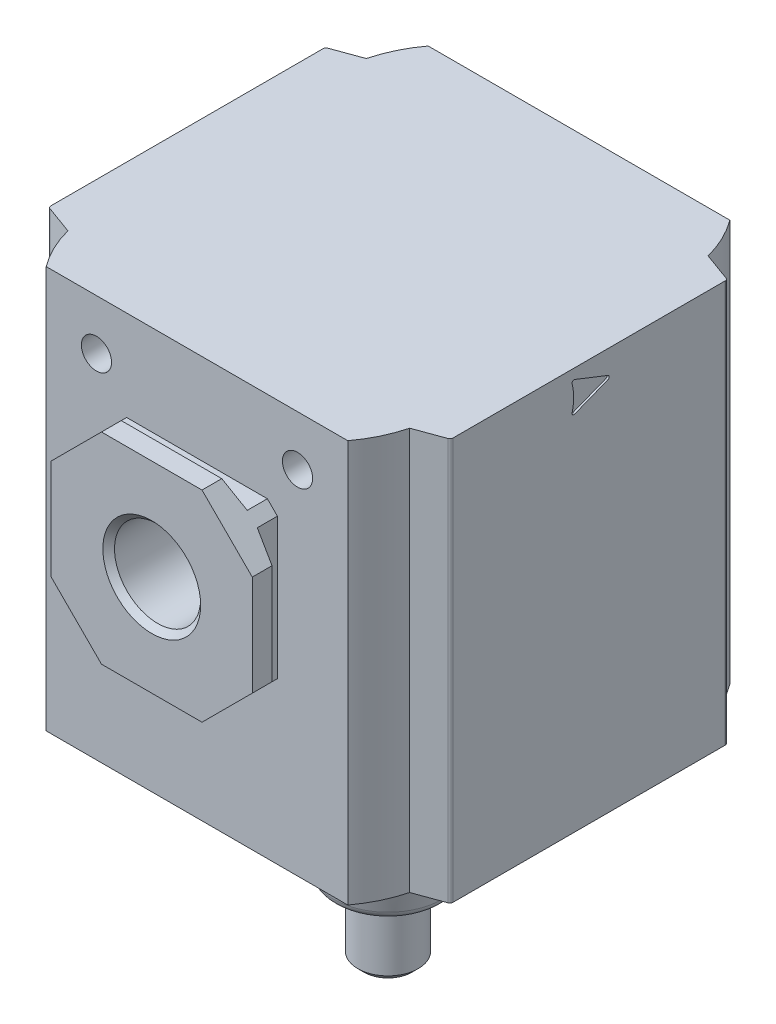
from build123d import *

# Parameters (mm, degrees)
EXTRUDE_1_DEPTH          = 40
EXTRUDE_2_DEPTH          = 40
EXTRUDE_3_DEPTH          = 40
EXTRUDE_4_DEPTH          = 2
EXTRUDE_5_DEPTH          = 2.5
CUT_EXTRUDE_1_DEPTH      = 10
CUT_EXTRUDE_1_DEPTH_BACK = 10
CUT_EXTRUDE_2_DEPTH      = 10
CUT_EXTRUDE_2_DEPTH_BACK = 10
CUT_EXTRUDE_3_DEPTH      = 10
CUT_EXTRUDE_3_DEPTH_BACK = 10
CUT_EXTRUDE_4_DEPTH      = 10
CUT_EXTRUDE_4_DEPTH_BACK = 10
EXTRUDE_6_DEPTH          = 2
EXTRUDE_7_DEPTH          = 2.5
CUT_EXTRUDE_5_DEPTH      = 10
CUT_EXTRUDE_5_DEPTH_BACK = 10
CUT_EXTRUDE_6_DEPTH      = 10
CUT_EXTRUDE_6_DEPTH_BACK = 10
CUT_EXTRUDE_7_DEPTH      = 10
CUT_EXTRUDE_7_DEPTH_BACK = 10
CUT_EXTRUDE_8_DEPTH      = 10
CUT_EXTRUDE_8_DEPTH_BACK = 10
SKETCH_18_R              = 1.5
CUT_EXTRUDE_9_DEPTH      = 4
SKETCH_19_R              = 1.5
CUT_EXTRUDE_10_DEPTH     = 4
CUT_EXTRUDE_START        = -4
SKETCH_20_R              = 1.5
CUT_EXTRUDE_11_DEPTH     = 4
SKETCH_21_R              = 1.5
CUT_EXTRUDE_12_DEPTH     = 4
SKETCH_22_W              = 16.9585
SKETCH_22_H              = 11
CUT_EXTRUDE_13_DEPTH     = 0.2
CUT_EXTRUDE_START_2      = 0.2
CUT_EXTRUDE_14_DEPTH     = 0.2


with BuildPart() as part:
    # 草图1 → 凸台-拉伸1 (new body)
    with BuildSketch(Plane(origin=(0, 0, 0), x_dir=(1, 0, 0), z_dir=(0, 1, 0))):
        with BuildLine():
            Line((-17, 14.841910703), (-17, -14.841910703))
            ThreePointArc((-17, -14.841910703), (-16.201733132, -17.017987001), (-15, -19))
            Line((-15, -19), (15, -19))
            ThreePointArc((15, -19), (16.201733132, -17.017987001), (17, -14.841910703))
            Line((17, -14.841910703), (17, 14.841910703))
            ThreePointArc((17, 14.841910703), (16.201733132, 17.017987001), (15, 19))
            Line((15, 19), (-15, 19))
            ThreePointArc((-15, 19), (-16.201733132, 17.017987001), (-17, 14.841910703))
        make_face()
    extrude(amount=EXTRUDE_1_DEPTH)

    # 草图2 → 凸台-拉伸2 (add)
    with BuildSketch(Plane(origin=(0, 0, 0), x_dir=(1, 0, 0), z_dir=(0, 1, 0))):
        with BuildLine():
            Line((17, 14.841910703), (17, -14.841910703))
            Line((17, -14.841910703), (19.802606043, -13.821845525))
            ThreePointArc((19.802606043, -13.821845525), (19.945745613, -13.712010669), (20, -13.539937739))
            Line((20, -13.539937739), (20, 13.539937739))
            ThreePointArc((20, 13.539937739), (19.945745613, 13.712010669), (19.802606043, 13.821845525))
            Line((19.802606043, 13.821845525), (17, 14.841910703))
        make_face()
    extrude(amount=EXTRUDE_2_DEPTH)

    # 草图3 → 凸台-拉伸3 (add)
    with BuildSketch(Plane(origin=(0, 0, 0), x_dir=(1, 0, 0), z_dir=(0, 1, 0))):
        with BuildLine():
            Line((-19.802606043, -13.821845525), (-17, -14.841910703))
            Line((-17, -14.841910703), (-17, 14.841910703))
            Line((-17, 14.841910703), (-19.802606043, 13.821845525))
            ThreePointArc((-19.802606043, 13.821845525), (-19.945745613, 13.712010669), (-20, 13.539937739))
            Line((-20, 13.539937739), (-20, -13.539937739))
            ThreePointArc((-20, -13.539937739), (-19.945745613, -13.712010669), (-19.802606043, -13.821845525))
        make_face()
    extrude(amount=EXTRUDE_3_DEPTH)

    # 草图4 → 凸台-拉伸4 (add)
    with BuildSketch(Plane.XY.offset(-19)):
        Polygon((-8, 16), (-7, 15), (7, 15), (8, 16), (8, 30), (7, 31), (-7, 31), (-8, 30), align=None)
    extrude(amount=-EXTRUDE_4_DEPTH)

    # 草图5 → 凸台-拉伸5 (add)
    with BuildSketch(Plane.XY.offset(-21)):
        Polygon((-10, 18), (-5, 13), (5, 13), (10, 18), (10, 28), (5, 33), (-5, 33), (-10, 28), align=None)
    extrude(amount=-EXTRUDE_5_DEPTH)

    # 草图6 → 切除-拉伸1 (cut, two sides: drawn at the far end of the back side and taken through both)
    with BuildSketch(Plane(origin=(0, 0, 0), x_dir=(0, 0, -1), z_dir=(1, 0, 0)).offset(-CUT_EXTRUDE_1_DEPTH_BACK)):
        Polygon((21, 13), (21.535898385, 13), (21, 15), align=None)
    extrude(amount=CUT_EXTRUDE_1_DEPTH + CUT_EXTRUDE_1_DEPTH_BACK, mode=Mode.SUBTRACT)

    # 草图7 → 切除-拉伸2 (cut, two sides: drawn at the far end of the back side and taken through both)
    with BuildSketch(Plane(origin=(0, 0, 0), x_dir=(0, 0, -1), z_dir=(1, 0, 0)).offset(-CUT_EXTRUDE_2_DEPTH_BACK)):
        Polygon((21, 33), (21, 31), (21.535898385, 33), align=None)
    extrude(amount=CUT_EXTRUDE_2_DEPTH + CUT_EXTRUDE_2_DEPTH_BACK, mode=Mode.SUBTRACT)

    # 草图8 → 切除-拉伸3 (cut, two sides: drawn at the far end of the back side and taken through both)
    with BuildSketch(Plane(origin=(0, 23, 0), x_dir=(1, 0, 0), z_dir=(0, 1, 0)).offset(-CUT_EXTRUDE_3_DEPTH_BACK)):
        Polygon((8, 21), (10, 21), (10, 21.535898385), align=None)
    extrude(amount=CUT_EXTRUDE_3_DEPTH + CUT_EXTRUDE_3_DEPTH_BACK, mode=Mode.SUBTRACT)

    # 草图9 → 切除-拉伸4 (cut, two sides: drawn at the far end of the back side and taken through both)
    with BuildSketch(Plane(origin=(0, 23, 0), x_dir=(1, 0, 0), z_dir=(0, 1, 0)).offset(-CUT_EXTRUDE_4_DEPTH_BACK)):
        Polygon((-10, 21), (-8, 21), (-10, 21.535898385), align=None)
    extrude(amount=CUT_EXTRUDE_4_DEPTH + CUT_EXTRUDE_4_DEPTH_BACK, mode=Mode.SUBTRACT)

    # 草图10 → 凸台-拉伸6 (add)
    with BuildSketch(Plane.XY.offset(19)):
        Polygon((-8, 16), (-7, 15), (7, 15), (8, 16), (8, 30), (7, 31), (-7, 31), (-8, 30), align=None)
    extrude(amount=EXTRUDE_6_DEPTH)

    # 草图11 → 凸台-拉伸7 (add)
    with BuildSketch(Plane.XY.offset(21)):
        Polygon((-10, 18), (-5, 13), (5, 13), (10, 18), (10, 28), (5, 33), (-5, 33), (-10, 28), align=None)
    extrude(amount=EXTRUDE_7_DEPTH)

    # 草图12 → 切除-拉伸5 (cut, two sides: drawn at the far end of the back side and taken through both)
    with BuildSketch(Plane(origin=(0, 0, 0), x_dir=(0, 0, -1), z_dir=(1, 0, 0)).offset(-CUT_EXTRUDE_5_DEPTH_BACK)):
        Polygon((-21.535898385, 13), (-21, 13), (-21, 15), align=None)
    extrude(amount=CUT_EXTRUDE_5_DEPTH + CUT_EXTRUDE_5_DEPTH_BACK, mode=Mode.SUBTRACT)

    # 草图13 → 切除-拉伸6 (cut, two sides: drawn at the far end of the back side and taken through both)
    with BuildSketch(Plane(origin=(0, 0, 0), x_dir=(0, 0, -1), z_dir=(1, 0, 0)).offset(-CUT_EXTRUDE_6_DEPTH_BACK)):
        Polygon((-21.535898385, 33), (-21, 31), (-21, 33), align=None)
    extrude(amount=CUT_EXTRUDE_6_DEPTH + CUT_EXTRUDE_6_DEPTH_BACK, mode=Mode.SUBTRACT)

    # 草图14 → 切除-拉伸7 (cut, two sides: drawn at the far end of the back side and taken through both)
    with BuildSketch(Plane(origin=(0, 23, 0), x_dir=(1, 0, 0), z_dir=(0, 1, 0)).offset(-CUT_EXTRUDE_7_DEPTH_BACK)):
        Polygon((8, -21), (10, -21.535898385), (10, -21), align=None)
    extrude(amount=CUT_EXTRUDE_7_DEPTH + CUT_EXTRUDE_7_DEPTH_BACK, mode=Mode.SUBTRACT)

    # 草图15 → 切除-拉伸8 (cut, two sides: drawn at the far end of the back side and taken through both)
    with BuildSketch(Plane(origin=(0, 23, 0), x_dir=(1, 0, 0), z_dir=(0, 1, 0)).offset(-CUT_EXTRUDE_8_DEPTH_BACK)):
        Polygon((-10, -21), (-10, -21.535898385), (-8, -21), align=None)
    extrude(amount=CUT_EXTRUDE_8_DEPTH + CUT_EXTRUDE_8_DEPTH_BACK, mode=Mode.SUBTRACT)

    # 草图16 → 切除-旋转1 (revolve, cut)
    with BuildSketch(Plane(origin=(0, 0, 0), x_dir=(0, 0, -1), z_dir=(1, 0, 0)), mode=Mode.PRIVATE) as cut_revolve_1_sk:
        Polygon((23.5, 23), (23.5, 18.136), (22.919, 18.717), (13.5, 18.717), (13.5, 23), align=None)
    revolve(cut_revolve_1_sk.sketch.rotate(Axis((0, 23, -13.5), (0, 0, -1)), 90), axis=Axis((0, 23, -13.5), (0, 0, -1)), mode=Mode.SUBTRACT)

    # 草图17 → 切除-旋转2 (revolve, cut)
    with BuildSketch(Plane(origin=(0, 0, 0), x_dir=(0, 0, -1), z_dir=(1, 0, 0)), mode=Mode.PRIVATE) as cut_revolve_2_sk:
        Polygon((-23.5, 23), (-23.5, 27.864), (-22.919, 27.283), (-13.5, 27.283), (-13.5, 23), align=None)
    revolve(cut_revolve_2_sk.sketch.rotate(Axis((0, 23, 13.5), (0, 0, 1)), 270), axis=Axis((0, 23, 13.5), (0, 0, 1)), mode=Mode.SUBTRACT)

    # 草图18 → 切除-拉伸9 (cut)
    with BuildSketch(Plane.XY.offset(-19)):
        with Locations((-10, 35)):
            Circle(SKETCH_18_R)
    extrude(amount=CUT_EXTRUDE_9_DEPTH, mode=Mode.SUBTRACT)

    # 草图19 → 切除-拉伸10 (cut)
    with BuildSketch(Plane.XY.offset(-19)):
        with Locations((10, 35)):
            Circle(SKETCH_19_R)
    extrude(amount=CUT_EXTRUDE_10_DEPTH, mode=Mode.SUBTRACT)

    # 草图20 → 切除-拉伸11 (cut)
    with BuildSketch(Plane.XY.offset(19).offset(CUT_EXTRUDE_START)):
        with Locations((-10, 35)):
            Circle(SKETCH_20_R)
    extrude(amount=CUT_EXTRUDE_11_DEPTH, mode=Mode.SUBTRACT)

    # 草图21 → 切除-拉伸12 (cut)
    with BuildSketch(Plane.XY.offset(19).offset(CUT_EXTRUDE_START)):
        with Locations((10, 35)):
            Circle(SKETCH_21_R)
    extrude(amount=CUT_EXTRUDE_12_DEPTH, mode=Mode.SUBTRACT)

    # 草图22 → 切除-旋转3 (revolve, cut)
    with BuildSketch(Plane(origin=(0, 0, 0), x_dir=(0, 0, -1), z_dir=(1, 0, 0)), mode=Mode.PRIVATE) as cut_revolve_3_sk:
        with Locations((8.47925, 5.5)):
            Rectangle(SKETCH_22_W, SKETCH_22_H)
    revolve(cut_revolve_3_sk.sketch.rotate(Axis((0, 0, 0), (0, 1, 0)), 180), axis=Axis((0, 0, 0), (0, 1, 0)), mode=Mode.SUBTRACT)

    # 草图23 → 旋转1 (revolve)
    with BuildSketch(Plane(origin=(0, 0, 0), x_dir=(0, 0, -1), z_dir=(1, 0, 0)), mode=Mode.PRIVATE) as revolve_1_sk:
        with BuildLine():
            Line((0, 11), (9.25, 11))
            ThreePointArc((9.25, 11), (10.310660172, 10.560660172), (10.75, 9.5))
            Line((10.75, 9.5), (10.75, 9.1))
            Line((10.75, 9.1), (13.35, 9.1))
            Line((13.35, 9.1), (13.35, 5.5))
            Line((13.35, 5.5), (7.7, 5.5))
            Line((7.7, 5.5), (7.7, -2.5))
            Line((7.7, -2.5), (5.41229688, -13.798452142))
            ThreePointArc((5.41229688, -13.798452142), (5.065253382, -14.374096939), (4.432186301, -14.6))
            Line((4.432186301, -14.6), (3, -14.6))
            Line((3, -14.6), (3, -20.9865))
            Line((3, -20.9865), (2.3865, -21.6))
            Line((2.3865, -21.6), (1.5, -21.6))
            Line((1.5, -21.6), (1.5, -16.8))
            ThreePointArc((1.5, -16.8), (1.441421356, -16.658578644), (1.3, -16.6))
            Line((1.3, -16.6), (0, -16.6))
            Line((0, -16.6), (0, 11))
        make_face()
    revolve(revolve_1_sk.sketch.rotate(Axis((0, -21.6, 0), (0, 1, 0)), 180), axis=Axis((0, -21.6, 0), (0, 1, 0)))

    # 草图24 → 切除-拉伸13 (cut)
    with BuildSketch(Plane(origin=(20, 0, 0), x_dir=(0, 0, -1), z_dir=(1, 0, 0))):
        with BuildLine():
            Line((-1.426695096, 36.013918321), (1.873304904, 37.313918321))
            ThreePointArc((1.873304904, 37.313918321), (2, 37.5), (1.873304904, 37.686081679))
            Line((1.873304904, 37.686081679), (-1.426695096, 38.986081679))
            ThreePointArc((-1.426695096, 38.986081679), (-1.612558916, 38.965319359), (-1.7, 38.8))
            ThreePointArc((-1.7, 38.8), (-1.528043082, 37.5), (-1.7, 36.2))
            ThreePointArc((-1.7, 36.2), (-1.612558916, 36.034680641), (-1.426695096, 36.013918321))
        make_face()
    extrude(amount=-CUT_EXTRUDE_13_DEPTH, mode=Mode.SUBTRACT)

    # 草图25 → 切除-拉伸14 (cut)
    with BuildSketch(Plane(origin=(-20, 0, 0), x_dir=(0, 0, -1), z_dir=(1, 0, 0)).offset(CUT_EXTRUDE_START_2)):
        with BuildLine():
            Line((-1.426695096, 36.013918321), (1.873304904, 37.313918321))
            ThreePointArc((1.873304904, 37.313918321), (2, 37.5), (1.873304904, 37.686081679))
            Line((1.873304904, 37.686081679), (-1.426695096, 38.986081679))
            ThreePointArc((-1.426695096, 38.986081679), (-1.612558916, 38.965319359), (-1.7, 38.8))
            ThreePointArc((-1.7, 38.8), (-1.528043082, 37.5), (-1.7, 36.2))
            ThreePointArc((-1.7, 36.2), (-1.612558916, 36.034680641), (-1.426695096, 36.013918321))
        make_face()
    extrude(amount=-CUT_EXTRUDE_14_DEPTH, mode=Mode.SUBTRACT)


solid = part.part
